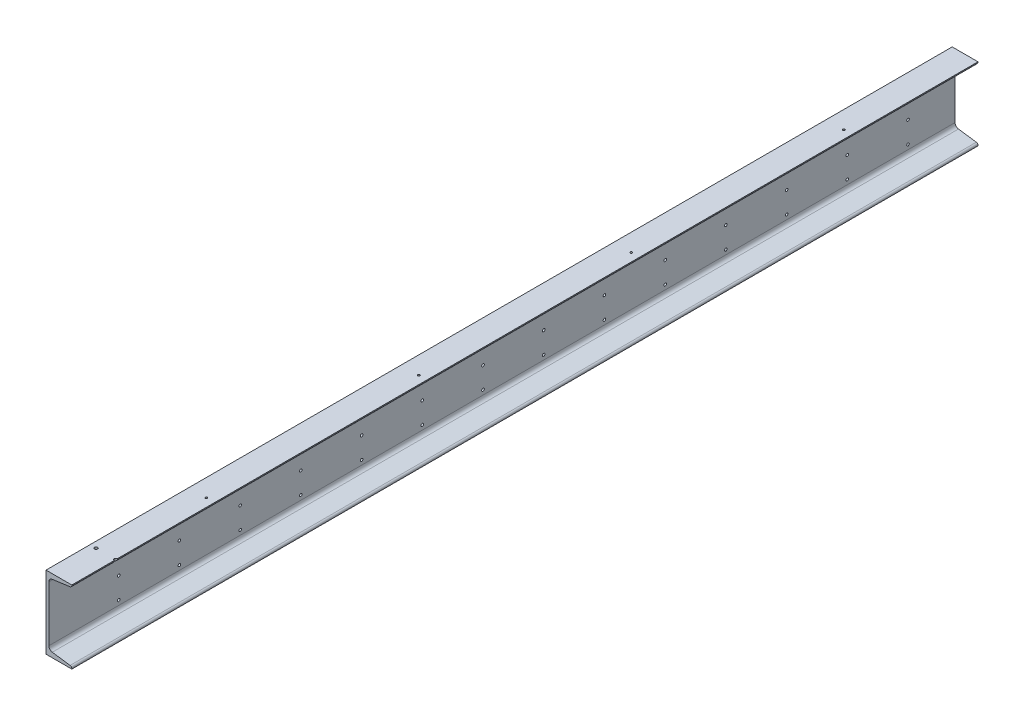
SolidWorks part; units mm, degrees
material "1023 碳钢板 (SS)"
ref_plane "前视基准面" through (0, 0, 0) normal (0, 0, 1) x (1, 0, 0)
ref_plane "上视基准面" through (0, 0, 0) normal (0, 1, 0) x (1, 0, 0)
ref_plane "右视基准面" through (0, 0, 0) normal (1, 0, 0) x (0, 0, -1)
sketch "草图1" plane through (0, 0, 0) normal (0, 0, 1) x (1, 0, 0)
  line L0 (0, 0) -> (-85, 0)
  line L1 (-85, 0) -> (-85, -240)
  line L2 (-85, -240) -> (0, -240)
  line L3 (0, -240) -> (0, -238.6233)
  line L4 (-5.5954, -232.1866) -> (-64.3093, -223.9349)
  line L5 (-75.5, -211.0614) -> (-75.5, -28.9386)
  line L6 (-64.3093, -16.0651) -> (-5.5954, -7.8134)
  line L7 (0, -1.3767) -> (0, 0)
  line L8 (-42.5, -227) -> (-42.5, -240) construction
  arc A0 (-64.3093, -223.9349) -> (-75.5, -211.0614) centre (-62.5, -211.0614) cw
  arc A1 (-75.5, -28.9386) -> (-64.3093, -16.0651) centre (-62.5, -28.9386) cw
  arc A2 (0, -238.6233) -> (-5.5954, -232.1866) centre (-6.5, -238.6233) ccw
  arc A3 (-5.5954, -7.8134) -> (0, -1.3767) centre (-6.5, -1.3767) ccw
  dimension "D7" = 13
  dimension "D8" = 6.5
  dimension "D1" = 240
  dimension "D2" = 85
  dimension "D3" = 42.5
  dimension "D4" = 13
  dimension "D5" = 9.5
  dimension "D6" = 8
extrude "凸台-拉伸1" add sketch "草图1" along normal blind 2985 contours A3 L6 A1 L5 A0 L4 A2 L3 L2 L1 L0 L7
sketch "草图2" plane through (-85, 0, 0) normal (-1, 0, 0) x (0, 0, 1)
  line L0 (2985, 0) -> (0, 0) construction
  line L2 (0, 0) -> (0, -240) construction
  circle A0 centre (2755, -126) radius 10
  circle A1 centre (2755, -196) radius 10
  circle A2 centre (2555, -126) radius 10
  circle A3 centre (2555, -196) radius 10
  circle A4 centre (2355, -126) radius 10
  circle A5 centre (2355, -196) radius 10
  circle A6 centre (2155, -126) radius 10
  circle A7 centre (2155, -196) radius 10
  circle A8 centre (1955, -126) radius 10
  circle A9 centre (1955, -196) radius 10
  circle A10 centre (1755, -126) radius 10
  circle A11 centre (1755, -196) radius 10
  circle A12 centre (1555, -126) radius 10
  circle A13 centre (1555, -196) radius 10
  circle A14 centre (1355, -126) radius 10
  circle A15 centre (1355, -196) radius 10
  circle A16 centre (1155, -126) radius 10
  circle A17 centre (1155, -196) radius 10
  circle A18 centre (955, -126) radius 10
  circle A19 centre (955, -196) radius 10
  circle A20 centre (755, -126) radius 10
  circle A21 centre (755, -196) radius 10
  circle A22 centre (555, -126) radius 10
  circle A23 centre (555, -196) radius 10
  circle A24 centre (355, -126) radius 10
  circle A25 centre (355, -196) radius 10
  circle A26 centre (155, -126) radius 10
  circle A27 centre (155, -196) radius 10
  dimension "D3" = 155
  dimension "D4" = 20
  dimension "D1" = 70
  dimension "D2" = 126
  dimension "D5" = 14
hole_wizard "M10 螺纹孔2" positions "草图5" profile "草图6" tap size "M10" standard "ISO"
sketch "草图5" plane through (-85, 0, 0) normal (-1, 0, 0) x (0, 0, 1)
  point P0 (155, -126)
  point P3 (155, -196)
  point P6 (355, -126)
  point P9 (355, -196)
  point P12 (555, -126)
  point P15 (555, -196)
  point P18 (755, -126)
  point P21 (755, -196)
  point P24 (955, -126)
  point P27 (955, -196)
  point P30 (1155, -126)
  point P33 (1155, -196)
  point P36 (1355, -126)
  point P39 (1355, -196)
  point P42 (1555, -196)
  point P45 (1555, -126)
  point P48 (1755, -196)
  point P51 (1755, -126)
  point P54 (1955, -126)
  point P57 (1955, -196)
  point P60 (2155, -196)
  point P63 (2155, -126)
  point P66 (2355, -126)
  point P69 (2355, -196)
  point P72 (2555, -196)
  point P75 (2555, -126)
  point P78 (2755, -126)
  point P81 (2755, -196)
sketch "草图6" plane through (-85, -126, 155) normal (0, 1, 0) x (0, 0, 1)
  line L0 (0, 0) -> (0, 27.0537)
  line L1 (0, 27.0537) -> (4.25, 24.5)
  line L2 (4.25, 24.5) -> (4.25, 0)
  line L5 (4.25, 0) -> (0, 0)
  line L10 (0, 27.0537) -> (-4.25, 24.5) construction
  line L11 (0, -6.35) -> (0, 107.95) construction
  dimension "螺纹孔钻头直径" = 8.5
  dimension "螺纹孔钻头深度" = 24.5
  dimension "导头角度" = 118
cosmetic thread "孔螺蚊线29" parameters "D1"=20, "D2"=10
cosmetic thread "孔螺蚊线30" parameters "D1"=20, "D2"=10
cosmetic thread "孔螺蚊线31" parameters "D1"=20, "D2"=10
cosmetic thread "孔螺蚊线32" parameters "D1"=20, "D2"=10
cosmetic thread "孔螺蚊线33" parameters "D1"=20, "D2"=10
cosmetic thread "孔螺蚊线34" parameters "D1"=20, "D2"=10
cosmetic thread "孔螺蚊线35" parameters "D1"=20, "D2"=10
cosmetic thread "孔螺蚊线36" parameters "D1"=20, "D2"=10
cosmetic thread "孔螺蚊线37" parameters "D1"=20, "D2"=10
cosmetic thread "孔螺蚊线38" parameters "D1"=20, "D2"=10
cosmetic thread "孔螺蚊线39" parameters "D1"=20, "D2"=10
cosmetic thread "孔螺蚊线40" parameters "D1"=20, "D2"=10
cosmetic thread "孔螺蚊线41" parameters "D1"=20, "D2"=10
cosmetic thread "孔螺蚊线42" parameters "D1"=20, "D2"=10
cosmetic thread "孔螺蚊线43" parameters "D1"=20, "D2"=10
cosmetic thread "孔螺蚊线44" parameters "D1"=20, "D2"=10
cosmetic thread "孔螺蚊线45" parameters "D1"=20, "D2"=10
cosmetic thread "孔螺蚊线46" parameters "D1"=20, "D2"=10
cosmetic thread "孔螺蚊线47" parameters "D1"=20, "D2"=10
cosmetic thread "孔螺蚊线48" parameters "D1"=20, "D2"=10
cosmetic thread "孔螺蚊线49" parameters "D1"=20, "D2"=10
cosmetic thread "孔螺蚊线50" parameters "D1"=20, "D2"=10
cosmetic thread "孔螺蚊线51" parameters "D1"=20, "D2"=10
cosmetic thread "孔螺蚊线52" parameters "D1"=20, "D2"=10
cosmetic thread "孔螺蚊线53" parameters "D1"=20, "D2"=10
cosmetic thread "孔螺蚊线54" parameters "D1"=20, "D2"=10
cosmetic thread "孔螺蚊线55" parameters "D1"=20, "D2"=10
cosmetic thread "孔螺蚊线56" parameters "D1"=20, "D2"=10
sketch "草图8" plane through (0, 0, 0) normal (0, 1, 0) x (1, 0, 0)
  line L0 (0, 0) -> (-85, 0) construction
  line L3 (0, -2985) -> (0, 0) construction
  circle A0 centre (-27, -415) radius 6
  circle A1 centre (-27, -1815) radius 20.8625
  circle A2 centre (-27, -1115) radius 25.1147
  circle A3 centre (-27, -2515) radius 19.3987
  dimension "D6" = 12
  dimension "D1" = 415
  dimension "D2" = 1115
  dimension "D3" = 1815
  dimension "D4" = 2515
  dimension "D5" = 27
hole_wizard "M8 螺纹孔1" positions "草图9" profile "草图10" tap size "M8" standard "ISO"
sketch "草图9" plane through (0, 0, 0) normal (0, 1, 0) x (1, 0, 0)
  point P0 (-27, -415)
  point P3 (-27, -1115)
  point P6 (-27, -1815)
  point P9 (-27, -2515)
sketch "草图10" plane through (-27, 0, 415) normal (1, 0, 0) x (0, 0, 1)
  line L0 (0, 0) -> (0, 21.7929)
  line L1 (0, 21.7929) -> (3.4, 19.75)
  line L2 (3.4, 19.75) -> (3.4, 0)
  line L5 (3.4, 0) -> (0, 0)
  line L10 (0, 21.7929) -> (-3.4, 19.75) construction
  line L11 (0, -6.35) -> (0, 107.95) construction
  dimension "螺纹孔钻头直径" = 6.8
  dimension "螺纹孔钻头深度" = 19.75
  dimension "导头角度" = 118
cosmetic thread "孔螺蚊线57" parameters "D1"=16, "D2"=8
cosmetic thread "孔螺蚊线58" parameters "D1"=16, "D2"=8
cosmetic thread "孔螺蚊线59" parameters "D1"=16, "D2"=8
cosmetic thread "孔螺蚊线60" parameters "D1"=16, "D2"=8
sketch "草图11" plane through (0, 0, 0) normal (0, 1, 0) x (1, 0, 0)
  line L0 (0, -2985) -> (0, 0) construction
  line L1 (0, 0) -> (-85, 0) construction
  circle A0 centre (0, -2840) radius 13.0818
  circle A1 centre (-65, -2840) radius 10.9987
  dimension "D2" = 2840
  dimension "D1" = 65
hole_wizard "M12 螺纹孔1" positions "草图12" profile "草图13" tap size "M12" standard "ISO"
sketch "草图12" plane through (0, 0, 0) normal (0, 1, 0) x (1, 0, 0)
  point P0 (-65, -2840)
  point P3 (0, -2840)
sketch "草图13" plane through (-65, 0, 2840) normal (1, 0, 0) x (0, 0, 1)
  line L0 (0, 0) -> (0, 32.3144)
  line L1 (0, 32.3144) -> (5.1, 29.25)
  line L2 (5.1, 29.25) -> (5.1, 0)
  line L5 (5.1, 0) -> (0, 0)
  line L10 (0, 32.3144) -> (-5.1, 29.25) construction
  line L11 (0, -6.35) -> (0, 107.95) construction
  dimension "螺纹孔钻头直径" = 10.2
  dimension "螺纹孔钻头深度" = 29.25
  dimension "导头角度" = 118
cosmetic thread "孔螺蚊线61" parameters "D1"=24, "D2"=12
sketch "草图14" plane through (-85, 0, 0) normal (-1, 0, 0) x (0, 0, 1)
  line L0 (2985, 0) -> (0, 0) construction
  line L1 (0, 0) -> (0, -240) construction
  circle A0 centre (1600, -50) radius 22.5
  dimension "D1" = 45
  dimension "D3" = 1600
  dimension "D2" = 50
extrude "切除-拉伸1" cut sketch "草图14" against normal blind 10
